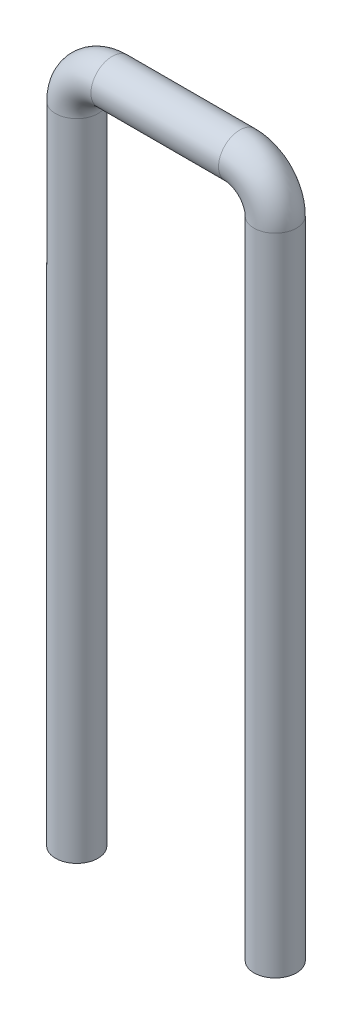
SolidWorks part; units mm, degrees
ref_plane "前视基准面" through (0, 0, 0) normal (0, 0, 1) x (1, 0, 0)
ref_plane "上视基准面" through (0, 0, 0) normal (0, 1, 0) x (1, 0, 0)
ref_plane "右视基准面" through (0, 0, 0) normal (1, 0, 0) x (0, 0, -1)
sketch "草图1" plane through (0, 0, 0) normal (0, 0, 1) x (1, 0, 0)
  line L0 (0, 171.4654) -> (0, -88.4577) construction
  line L1 (-14, 0) -> (-14, 91)
  line L2 (-9, 96) -> (9, 96)
  line L3 (14, 91) -> (14, 0)
  arc A0 (14, 91) -> (9, 96) centre (9, 91) ccw
  arc A1 (-9, 96) -> (-14, 91) centre (-9, 91) ccw
  point P9 (14, 96)
  point P12 (-14, 96)
  dimension "D3" = 5
  dimension "D1" = 28
  dimension "D2" = 96
sketch "草图2" plane through (0, 0, 0) normal (0, 1, 0) x (1, 0, 0)
  line L0 (-9, 0) -> (9, 0) construction
  circle A0 centre (-14, 0) radius 3
  dimension "D1" = 6
sweep "扫描1" add profiles "草图2" path "草图1"
cosmetic thread "装饰螺纹线1" parameters "D1"=46, "D2"=5
cosmetic thread "装饰螺纹线2" parameters "D1"=46, "D2"=5
